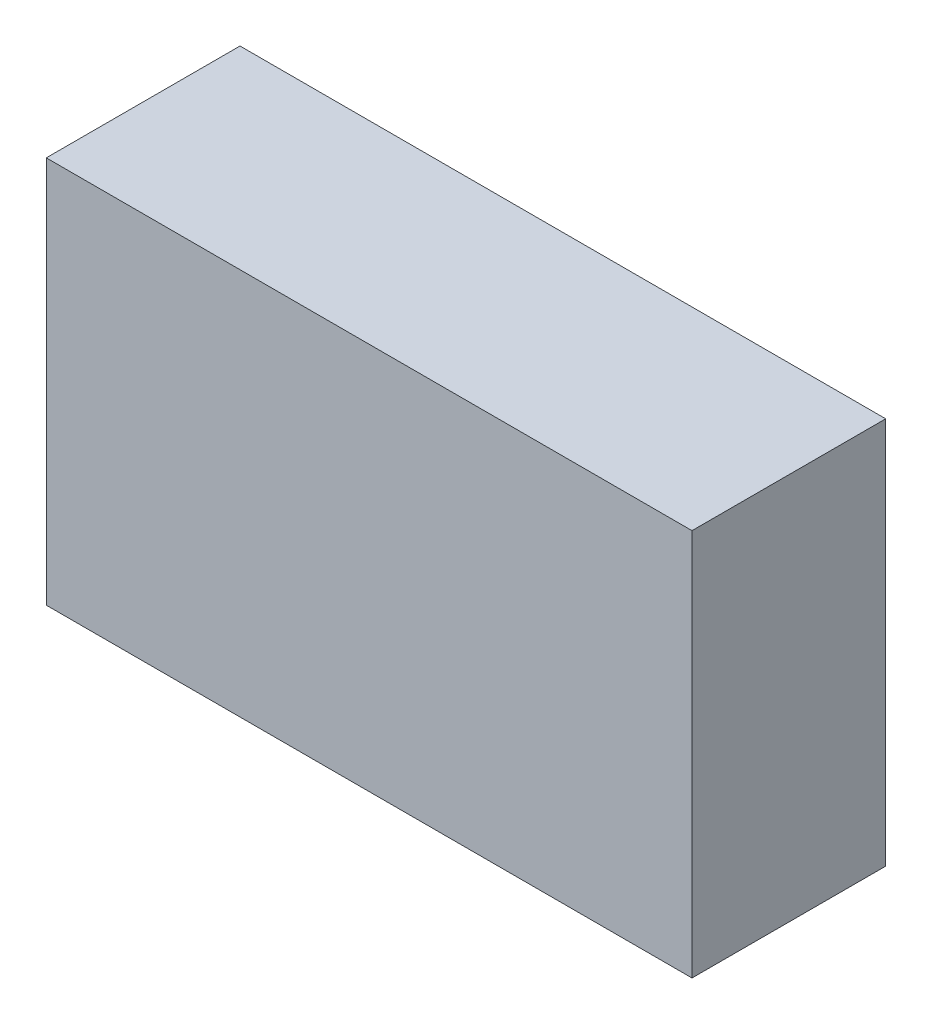
SolidWorks part; units mm, degrees
ref_plane "Front Plane" through (0, 0, 0) normal (0, 0, 1) x (1, 0, 0)
ref_plane "Top Plane" through (0, 0, 0) normal (0, 1, 0) x (1, 0, 0)
ref_plane "Right Plane" through (0, 0, 0) normal (1, 0, 0) x (0, 0, -1)
other "Configuration Table"
sketch "Sketch1" plane through (0, 0, 0) normal (0, 0, 1) x (1, 0, 0)
  line L1 (50, -30) -> (-50, -30)
  line L2 (50, -30) -> (50, 30)
  line L3 (50, 30) -> (-50, 30)
  line L4 (-50, -30) -> (-50, 30)
  line L5 (50, -30) -> (-50, 30) construction
  line L6 (50, 30) -> (-50, -30) construction
  point P0 (0, 0)
  dimension "D1" = 100
  dimension "D2" = 60
extrude "Boss-Extrude1" add sketch "Sketch1" along normal blind 30
